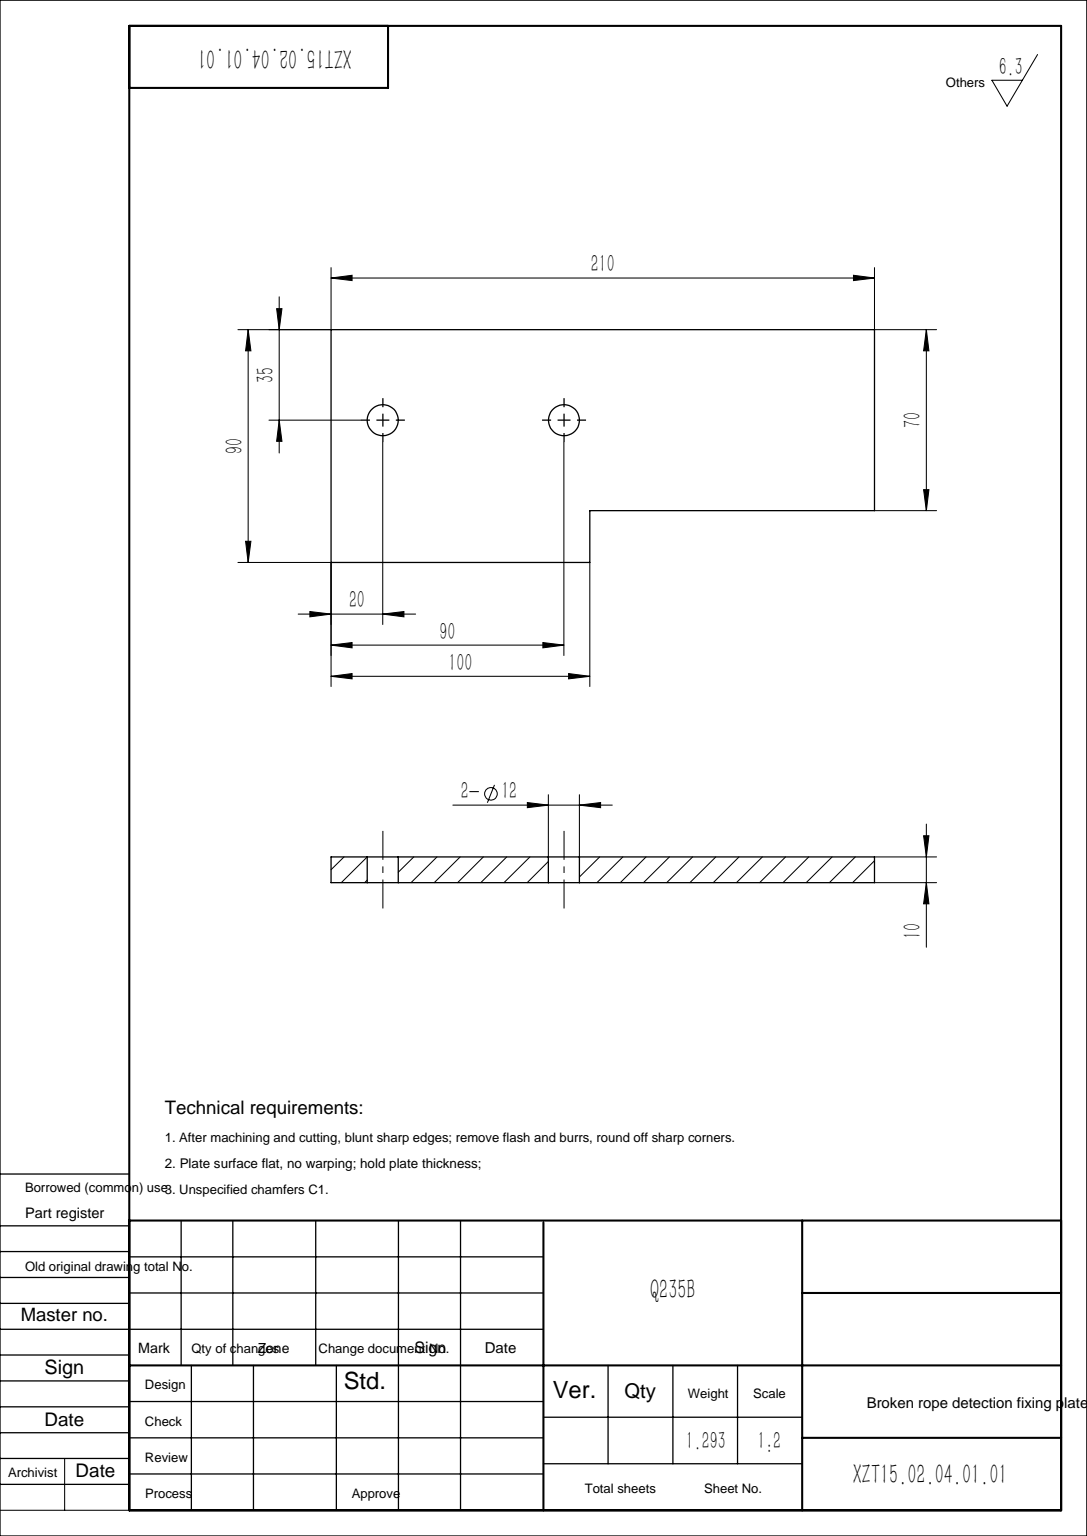
from build123d import *

# Parameters (mm, degrees)
BOSS_EXTRUDE1_DEPTH        = 5
F_12_0_12_DIAMETER_HOLE1_D = 12


with BuildPart() as part:
    # Sketch1 → Boss-Extrude1 (new, symmetric)
    with BuildSketch(Plane.XY):
        Polygon((0, 0), (0, 90), (210, 90), (210, 20), (100, 20), (100, 0), align=None)
    extrude(amount=BOSS_EXTRUDE1_DEPTH, both=True)

    # Ø12.0 (12) Diameter Hole1 (through all)
    with Locations(Plane.XY.offset(5)):
        with Locations((20, 55), (90, 55)):
            Hole(F_12_0_12_DIAMETER_HOLE1_D / 2)


solid = part.part
